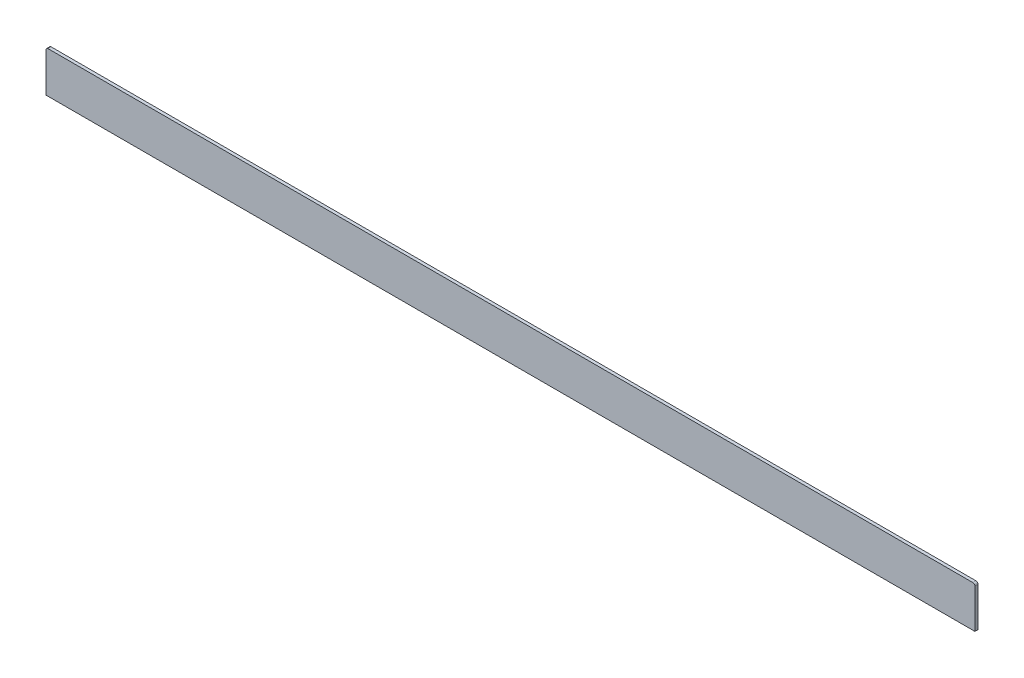
from build123d import *

# Parameters (mm, degrees)
SKETCH_1_W      = 900
SKETCH_1_H      = 40
EXTRUDE_1_DEPTH = 3
FILLET_1_R      = 2


with BuildPart() as part:
    # 草图1 → 凸台-拉伸1 (new body)
    with BuildSketch(Plane.XY):
        Rectangle(SKETCH_1_W, SKETCH_1_H)
    extrude(amount=EXTRUDE_1_DEPTH)

    # 圆角1
    fillet_1_edges = [part.edges().sort_by_distance(p)[0] for p in [
        (-450, 20, 1.5),
        (450, 20, 1.5),
    ]]
    fillet(fillet_1_edges, radius=FILLET_1_R)


solid = part.part
